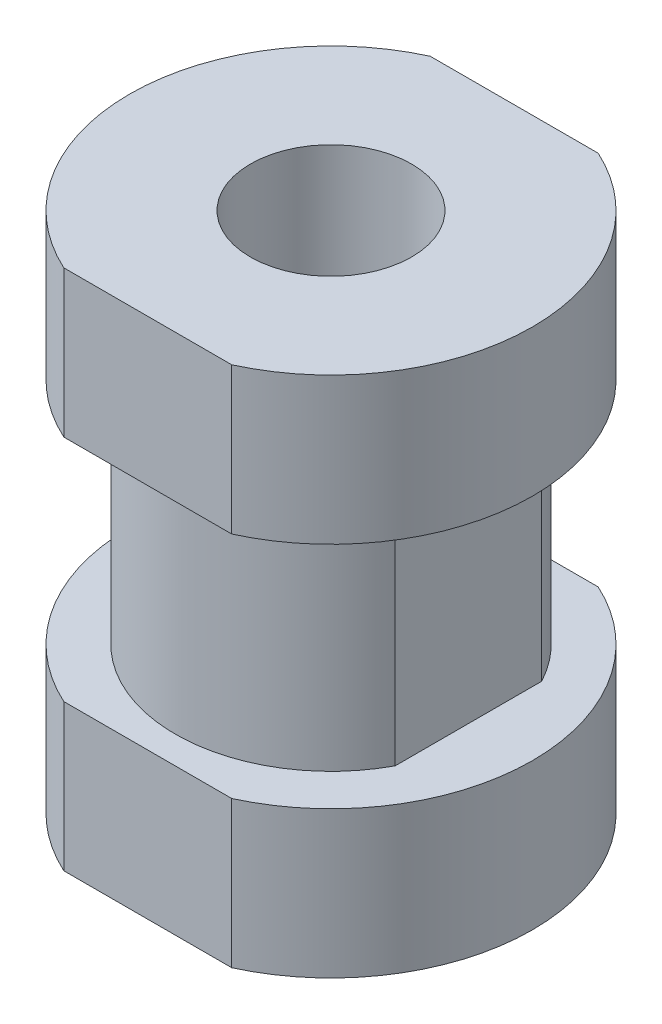
from build123d import *

# Parameters (mm, degrees)
SKETCH_1_R          = 11
EXTRUDE_1_DEPTH     = 4
SKETCH_2_R          = 8.5
EXTRUDE_2_DEPTH     = 12.5
EXTRUDE_START       = 8
SKETCH_9_R          = 11
EXTRUDE_3_DEPTH     = 8
M10X1_25_1_D        = 8.8
CUT_EXTRUDE_2_DEPTH = 33.46921619
SKETCH_10_W         = 1
SKETCH_10_H         = 12.5
CUT_EXTRUDE_3_DEPTH = 24.5


with BuildPart() as part:
    # 草图1 → 凸台-拉伸1 (new, symmetric)
    with BuildSketch(Plane(origin=(0, 0, 0), x_dir=(1, 0, 0), z_dir=(0, 1, 0))):
        with Locations(Location((0, 0, 0), (0, 0, 270))):
            Circle(SKETCH_1_R)
    extrude(amount=EXTRUDE_1_DEPTH, both=True)

    # 草图2 → 凸台-拉伸2 (add)
    with BuildSketch(Plane(origin=(0, 4, 0), x_dir=(1, 0, 0), z_dir=(0, 1, 0))):
        with Locations(Location((0, 0, 0), (0, 0, 270))):
            Circle(SKETCH_2_R)
    extrude(amount=EXTRUDE_2_DEPTH)

    # 草图9 → 凸台-拉伸3 (add)
    with BuildSketch(Plane(origin=(0, 16.5, 0), x_dir=(1, 0, 0), z_dir=(0, 1, 0)).offset(EXTRUDE_START)):
        with Locations(Location((0, 0, 0), (0, 0, 270))):
            Circle(SKETCH_9_R)
    extrude(amount=-EXTRUDE_3_DEPTH)

    # M10x1.25 螺纹孔1 (through all)
    with Locations(Plane(origin=(0, -4, 0), x_dir=(-1, 0, 0), z_dir=(0, -1, 0))):
        with Locations((0, 0)):
            Hole(M10X1_25_1_D / 2)

    # 草图6 → 切除-拉伸2 (cut, through all)
    with BuildSketch(Plane.XZ.offset(4)):
        with BuildLine():
            Line((-4.582575695, 10), (4.582575695, 10))
            ThreePointArc((4.582575695, 10), (0, 11), (-4.582575695, 10))
        make_face()
        with BuildLine():
            Line((-4.582575695, -10), (4.582575695, -10))
            ThreePointArc((4.582575695, -10), (0, -11), (-4.582575695, -10))
        make_face()
    extrude(amount=-CUT_EXTRUDE_2_DEPTH, mode=Mode.SUBTRACT)

    # 草图10 → 切除-拉伸3 (cut, symmetric)
    with BuildSketch(Plane.XY):
        with Locations((-8, 10.25)):
            Rectangle(SKETCH_10_W, SKETCH_10_H)
        with Locations((8, 10.25)):
            Rectangle(SKETCH_10_W, SKETCH_10_H)
    extrude(amount=CUT_EXTRUDE_3_DEPTH, both=True, mode=Mode.SUBTRACT)


solid = part.part
